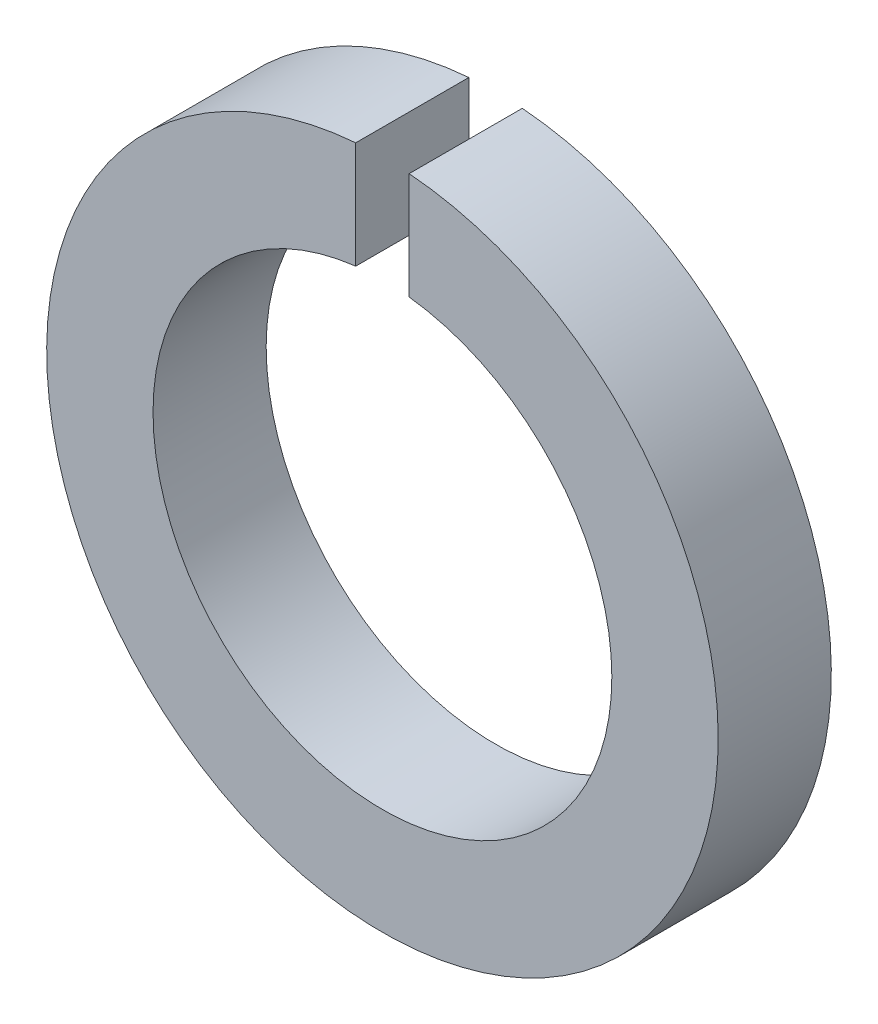
SolidWorks part; units mm, degrees
ref_plane "前视基准面" through (0, 0, 0) normal (0, 0, 1) x (1, 0, 0)
ref_plane "上视基准面" through (0, 0, 0) normal (0, 1, 0) x (1, 0, 0)
ref_plane "右视基准面" through (0, 0, 0) normal (1, 0, 0) x (0, 0, -1)
sketch "草图1" plane through (0, 0, 0) normal (0, 0, 1) x (1, 0, 0)
  line L0 (0, 0) -> (0, 103.5317) construction
  line L1 (-2.125, 26.6259) -> (-2.125, 18.1259)
  line L2 (2.125, 26.6259) -> (2.125, 18.1259)
  arc A0 (-2.125, 26.6259) -> (2.125, 26.6259) centre (0, 0) ccw
  arc A2 (-2.125, 18.1259) -> (2.125, 18.1259) centre (0, 0) ccw
extrude "拉伸1" add sketch "草图1" along normal blind 9
equation "\"D4@草图1\" = \"m@草图1\" / 2"
